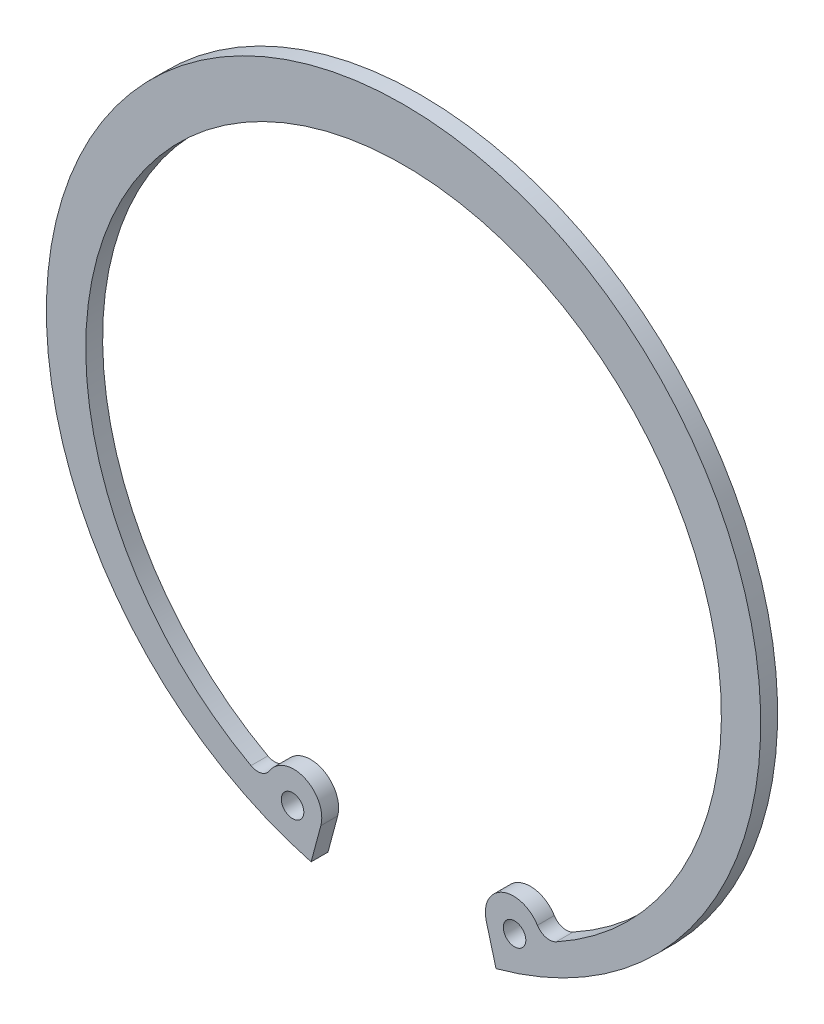
from build123d import *

# Parameters (mm, degrees)
BASE_EXTRUDE_DEPTH      = 1.5
BASE_EXTRUDE_DEPTH_BACK = 1.5
SKETCH1_R               = 2


with BuildPart() as part:
    # Sketch1 → Base-Extrude (new, two sides: drawn at the far end of the back side and taken through both)
    with BuildSketch(Plane.XY.offset(-BASE_EXTRUDE_DEPTH_BACK)):
        with BuildLine():
            Line((-14.708808387, -54.894020219), (-16.435009364, -61.336289969))
            ThreePointArc((-16.435009364, -61.336289969), (0, 63.5), (16.435009364, -61.336289969))
            Line((16.435009364, -61.336289969), (14.708808387, -54.894020219))
            ThreePointArc((14.708808387, -54.894020219), (17.560433321, -49.007812256), (23.796756449, -50.979482305))
            ThreePointArc((23.796756449, -50.979482305), (25.28518113, -52.085758206), (27.1261898, -51.862282302))
            ThreePointArc((27.1261898, -51.862282302), (0, 54.2), (-27.1261898, -51.862282302))
            ThreePointArc((-27.1261898, -51.862282302), (-25.28518113, -52.085758206), (-23.796756449, -50.979482305))
            ThreePointArc((-23.796756449, -50.979482305), (-17.560433321, -49.007812256), (-14.708808387, -54.894020219))
        make_face()
        with Locations((-19.733291854, -54.327131275)):
            Circle(SKETCH1_R, mode=Mode.SUBTRACT)
        with Locations(Location((19.733291854, -54.327131275, 0), (0, 0, 180))):
            Circle(SKETCH1_R, mode=Mode.SUBTRACT)
    extrude(amount=BASE_EXTRUDE_DEPTH + BASE_EXTRUDE_DEPTH_BACK)


solid = part.part
